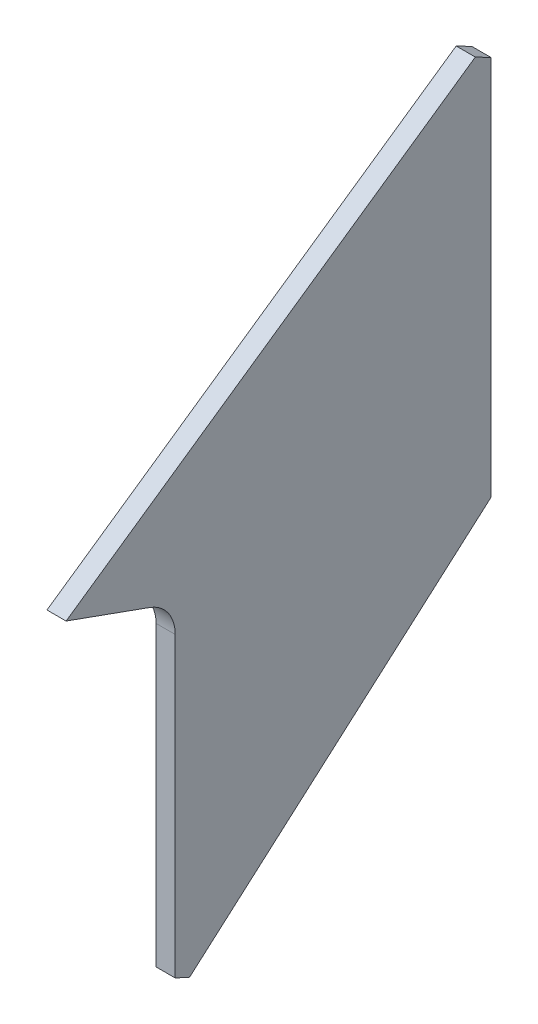
SolidWorks part; units mm, degrees
ref_plane "Front Plane" through (0, 0, 0) normal (0, 0, 1) x (1, 0, 0)
ref_plane "Top Plane" through (0, 0, 0) normal (0, 1, 0) x (1, 0, 0)
ref_plane "Right Plane" through (0, 0, 0) normal (1, 0, 0) x (0, 0, -1)
sketch "Sketch1" plane through (0, 0, 0) normal (1, 0, 0) x (0, 0, -1)
  line L0 (0, 145) -> (0, 344)
  line L1 (-8.2166, 348.3002) -> (-222, 200)
  line L2 (-222, 200) -> (-178.2315, 184.2587)
  line L3 (-165, 165.4388) -> (-165, 10)
  line L4 (-157.4884, 6.6011) -> (0, 145)
  line L5 (0, 344) -> (-8.2166, 348.3002)
  line L6 (-165, 10) -> (-157.4884, 6.6011)
  arc A0 (-178.2315, 184.2587) -> (-165, 165.4388) centre (-185, 165.4388) cw
  point P1 (0, 354)
  point P7 (-165, 0)
  point P9 (-165, 179.5)
  dimension "D8" = 20
  dimension "D1" = 354
  dimension "D2" = 165
  dimension "D3" = 145
  dimension "D4" = 179.5
  dimension "D5" = 200
  dimension "D6" = 222
  dimension "D7" = 179.5
extrude "Boss-Extrude1" add sketch "Sketch1" along normal blind 10
